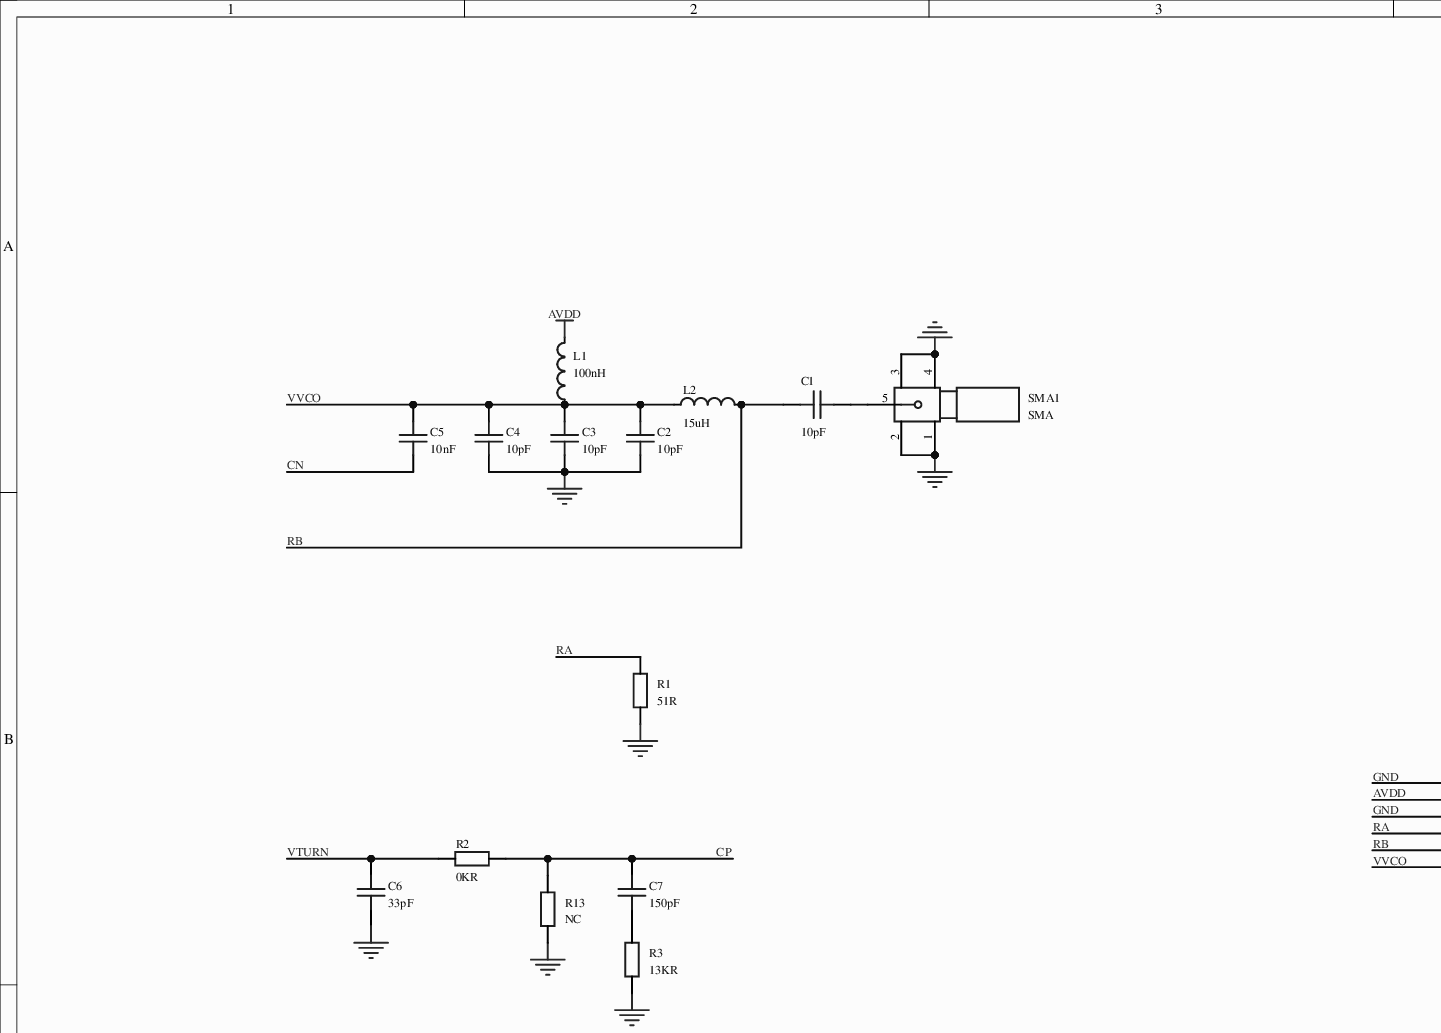
[diagram p0: MISC75048-3.schdoc, top left]
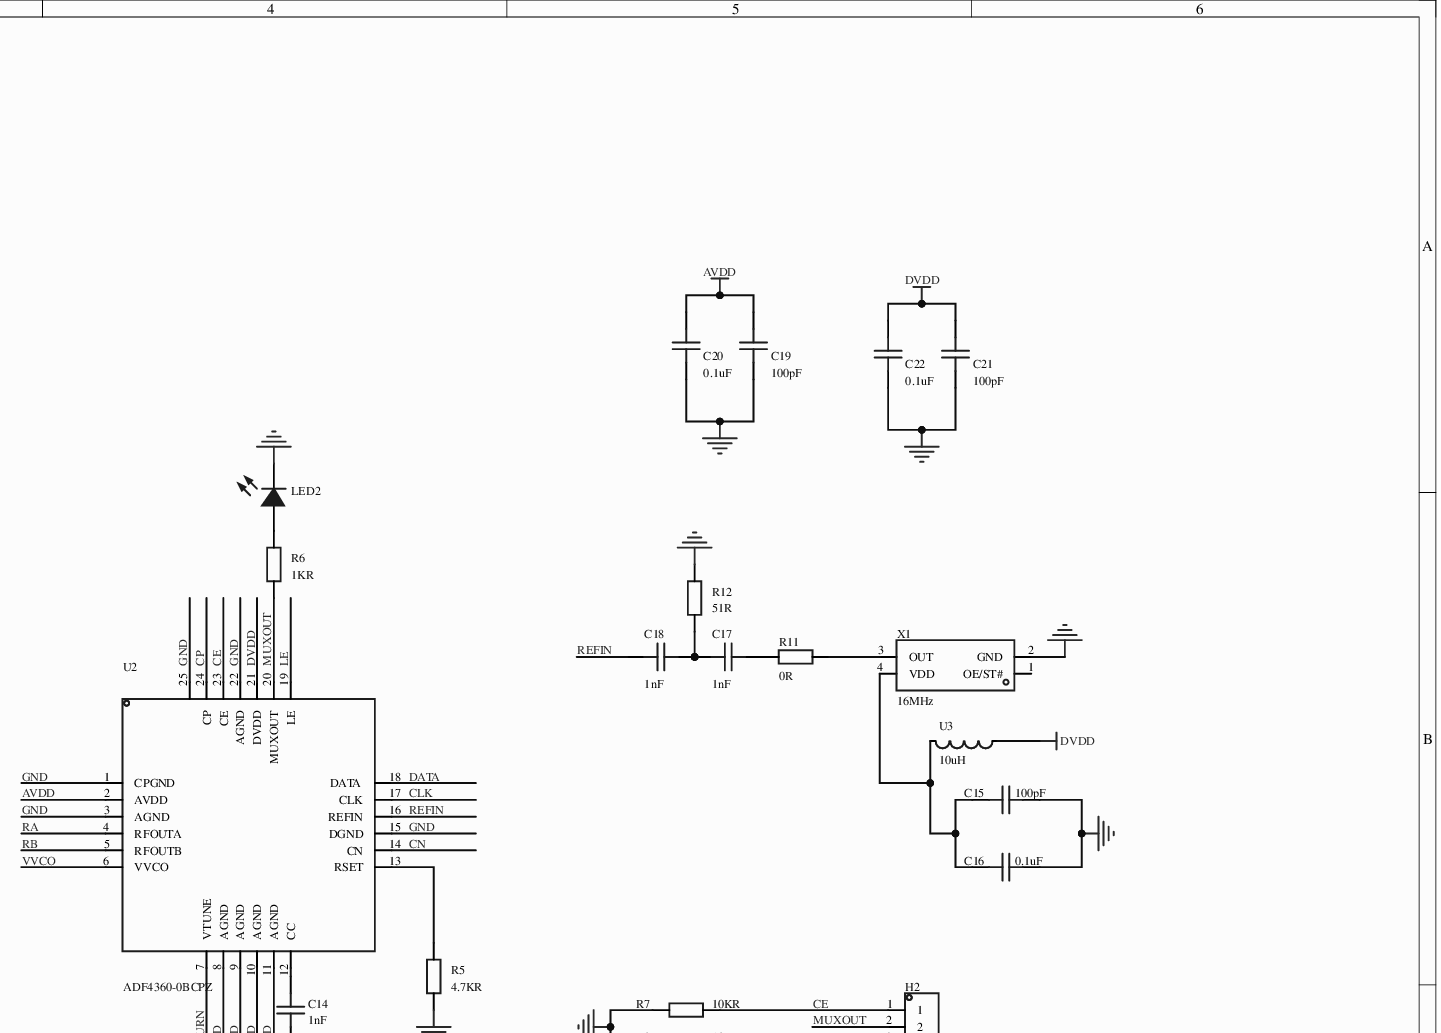
[diagram p1: MISC75048-3.schdoc, top right]
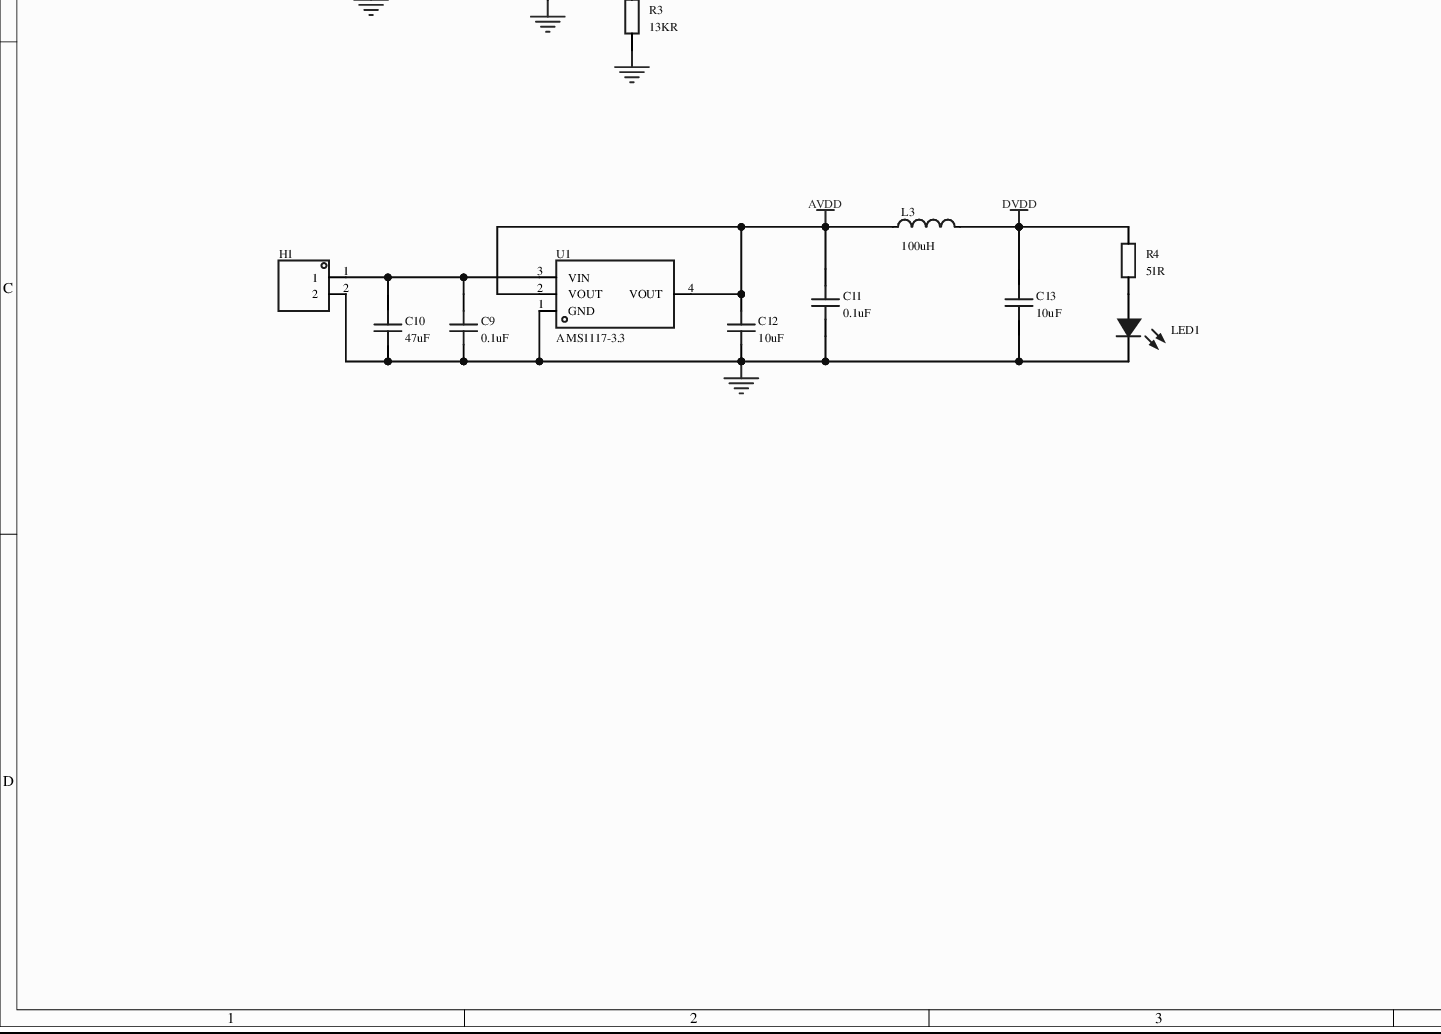
[diagram p2: MISC75048-3.schdoc, bottom left]
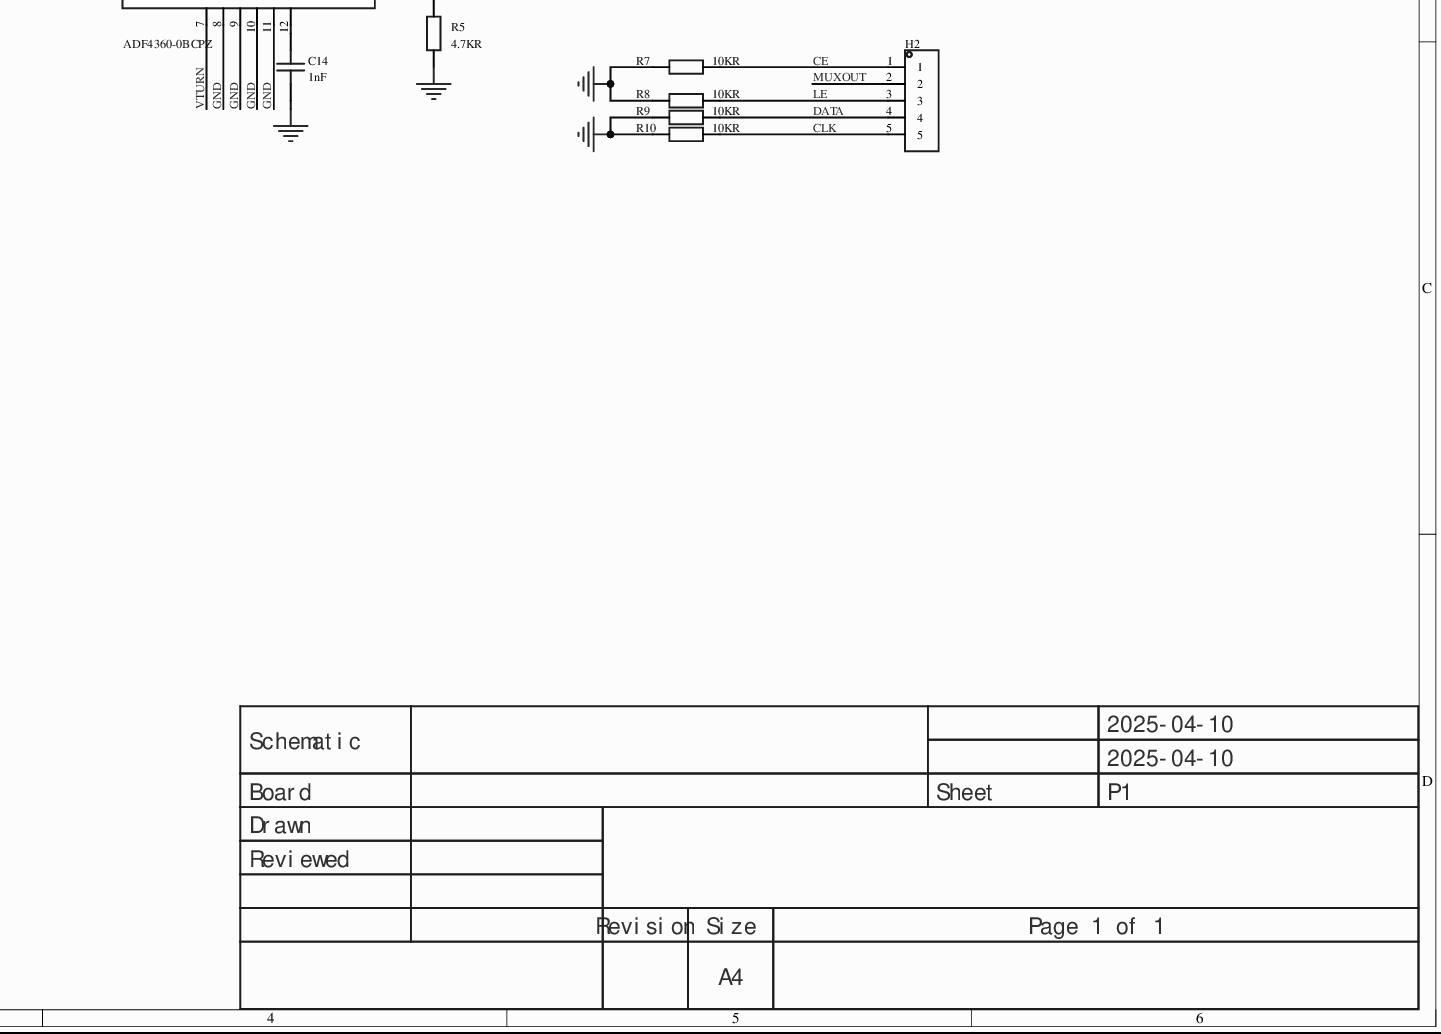
[diagram p3: MISC75048-3.schdoc, bottom right]
# Altium project MISC75048-2.PrjPcb
1 sheet, 46 parts. Net scope: global (net labels, ports and power ports of the same name join across sheets).
Board file: MISC75048.pcbdoc

## Sheet MISC75048-3.schdoc
size 420 x 297 mm; Version: V1.0; @Project Name: MISC75048; @Page Count: 1; @Update Date: 2025-04-10; @Create Date: 2025-04-10; @Schematic Name: MISC75048; @Page No: 1; @Create Time: 22:21:49; @Update Time: 22:48:33; @Board Name: MISC75048

### Parts
C1  10pF  [C0603]
C2  10pF  [C0603]
C3  10pF  [C0603]
C4  10pF  [C0603]
C5  10nF  [C0603]
C6  33pF  [C0603]
C7  150pF  [C0603]
C9  0.1uF  [C0603]
C10  47uF  [C0603]
C11  0.1uF  [C0603]
C12  10uF  [C0603]
C13  10uF  [C0603]
C14  1nF  [C0603]
C15  100pF  [C0603]
C16  0.1uF  [C0603]
C17  1nF  [C0603]
C18  1nF  [C0603]
C19  100pF  [C0603]
C20  0.1uF  [C0603]
C21  100pF  [C0603]
C22  0.1uF  [C0603]
H1  (no value)  [HDR-TH_2P-P2.54-V-M-1]
H2  (no value)  [HDR-TH_5P-P2.54-V-M]
L1  100nH  [L0805]
L2  15uH  [IND-SMD_L8.5-W8.0-LS9.5_ZEYH0850-15UH]
L3  100uH  [IND-SMD_L4.0-W4.0_SWPA4018S]
LED1  (no value)  [LED_0603]
LED2  (no value)  [LED_0603]
R1  51R  [R0603]
R2  0KR  [R0603]
R3  13KR  [R0603]
R4  51R  [R0603]
R5  4.7KR  [R0603]
R6  1KR  [R0603]
R7  10KR  [R0603]
R8  10KR  [R0603]
R9  10KR  [R0603]
R10  10KR  [R0603]
R11  0R  [R0603]
R12  51R  [R0603]
R13  NC  [R0603]
SMA1  SMA  [SMA-SMD_BWSMA-KE-P001]
U1  AMS1117-3.3  [SOT-223-3_L6.5-W3.4-P2.30-LS7.0-BR]
U2  ADF4360-0BCPZ  [LFCSP-24_L4.0-W4.0-P0.50-BL-EP2.3]
U3  10uH  [IND-SMD_L4.0-W4.0_LVF404015]
X1  16MHz  [OSC-SMD_4P-L7.0-W5.0-BL]

### Nets
AVDD: C11.2 C12.2 C19.2 C20.2 L1.2 L3.1 U1.2(VOUT) U1.4(VOUT) U2.2(AVDD)
DVDD: C13.2 C21.2 C22.2 L3.2 R4.2 U2.21(DVDD) U3.1
GND: C2.1 C3.1 C4.1 C6.1 C9.1 C10.1 C11.1 C12.1 C13.1 C14.1 C15.1 C16.1 C19.1 C20.1 C21.1 C22.1 H1.2 LED1.1(C) LED2.1(C) R1.1 R3.2 R5.1 R7.2 R8.2 R9.2 R10.2 R12.2 R13.2 SMA1.1 SMA1.2 SMA1.3 SMA1.4 U1.1(GND) U2.1(CPGND) U2.3(AGND) U2.8(AGND) U2.9(AGND) U2.10(AGND) U2.11(AGND) U2.15(DGND) U2.22(AGND) U2.25 X1.2(GND)
CE: H2.1 R7.1 U2.23(CE)
CLK: H2.5 R10.1 U2.17(CLK)
CN: C5.1 U2.14(CN)
CP: C7.2 R2.1 R13.1 U2.24(CP)
DATA: H2.4 R9.1 U2.18(DATA)
LE: H2.3 R8.1 U2.19(LE)
MUXOUT: H2.2 R6.2 U2.20(MUXOUT)
RA: R1.2 U2.4(RFOUTA)
RB: C1.1 L2.2 U2.5(RFOUTB)
REFIN: C18.2 U2.16(REFIN)
VTURN: C6.2 R2.2 U2.7(VTUNE)
VVCO: C2.2 C3.2 C4.2 C5.2 L1.1 L2.1 U2.6(VVCO)
NetC1_2: C1.2 SMA1.5
NetC7_1: C7.1 R3.1
NetC9_2: C9.2 C10.2 H1.1 U1.3(VIN)
NetC14_2: C14.2 U2.12(CC)
NetC15_2: C15.2 C16.2 U3.2 X1.4(VDD)
NetC17_1: C17.1 R11.1
NetC17_2: C17.2 C18.1 R12.1
NetLED1_2: LED1.2(A) R4.1
NetLED2_2: LED2.2(A) R6.1
NetR5_2: R5.2 U2.13(RSET)
NetR11_2: R11.2 X1.3(OUT)

Not connected (* = marked no-connect by the designer): X1 1(OE/ST#)*

### Notes on the sheet
- 2025-04-10
- Schematic
- Board
- Sheet
- P1
- Drawn
- Reviewed
- Revision
- Size
- A4
- Page 1 of 1

### Library data of the parts
C1-C7 C9-C22 = CAP_0603: ConvertToPcb: yes; SymbolName: CapAcitance; ModelId: ac125912035d415993ca9572d50418b1; ModelName: C0603_L1.6-W0.8-H0.8; ModelTransform: 62.992,31.496,0,0,0,0,0,0,0; Device: CAP_0603; AddInBom: yes; Supplier Footprint: 0603; FootprintName: C0603
  C1-C4: Value: 10pF
  C5: Value: 10nF
  C6: Value: 33pF
  C7: Value: 150pF
  C9 C11 C16 C20 C22: Value: 0.1uF
  C10: Value: 47uF
  C12 C13: Value: 10uF
  C14 C17 C18: Value: 1nF
  C15 C19 C21: Value: 100pF
H1 = HDR-M_2.54_1x2P: Symbol: 210S-1*2P L=11.6MMGold-plated black; ConvertToPcb: yes; ModelId: 79b2e9f2d70a4d68a1b7098f27c6d4c5; ModelName: HDR-M-2.54_1x2; ModelTransform: 200,100,0,0,0,0,0,0,-118.11; Device: HDR-M_2.54_1x2P; AddInBom: yes; SupplierPart: C124375; Supplier Footprint: 插件; FootprintName: HDR-TH_2P-P2.54-V-M-1
H2 = HDR-M_2.54_1x5P: Symbol: MTP125-1105S1; ConvertToPcb: yes; ModelId: 47d466e4a34f4fc5bc626cf773a24dd5; ModelName: HDR-TH_5P-P2.54-M-LI-1X5P; ModelTransform: 499.999,100,0,0,0,0,0,0,-118.11; Device: HDR-M_2.54_1x5P; AddInBom: yes; SupplierPart: C358687; Supplier Footprint: 插件; FootprintName: HDR-TH_5P-P2.54-V-M
L1 = SDFL2012LR10KTF: Inductance: 100nH; Tolerance: ±10%; Rated current: 250mA; Saturation current (Isat): -; DC resistance (DCR): 300mΩ;; Manufacturer: Sunlord(顺络); AddInBom: yes; ModelId: 37a81e68749a4138bd2dfa6897b24b85; ModelName: R0805_L2.0-W1.3-H0.6; ModelTransform: 78.74,51.181,0,0,0,0,0,0.001,0; Symbol: SDFL2012LR10KTF; Device: SDFL2012LR10KTF; LCSC Part Name: 100nH ±10%; SupplierPart: C74321; ManufacturerPart: SDFL2012LR10KTF; Supplier Footprint: 0805; Datasheet: example.com/upload/public/pdf/source/20231027/097A17DDB71564CE812E62F0F80142C9.pdf; Supplier: LCSC; ConvertToPcb: yes; FootprintName: L0805; Value: 100nH; Rated Current: 250mA; Saturation Current (Isat): -; DC Resistance (DCR): 300mΩ; Q @ Freq: -; Frequency - Self Resonant: -; Ratings: -
L2 = ZEYH0850-15UH: Inductance: 15uH; Tolerance: ±20%; Rated current: 5A; Saturation current (Isat): 9A; Type: molded integrated inductor;; Manufacturer: ZE(增益); AddInBom: yes; DC Resistance(DCR): 47mΩ; Symbol: ZEYH0850-15UH; Device: ZEYH0850-15UH; LCSC Part Name: 15uH ±20% 9A; SupplierPart: C45986904; ManufacturerPart: ZEYH0850-15UH; Supplier Footprint: SMD,8.5x8mm; Datasheet: example.com/upload/public/pdf/source/20250227/8D198FBC2D11620209AF2814C1FD1B5F.pdf; Supplier: LCSC; ConvertToPcb: yes; FootprintName: IND-SMD_L8.5-W8.0-LS9.5_ZEYH0850-15UH; Value: 15uH; Current Rating: 5A; Current - Saturation(Isat): 9A; Type: Molded integrated inductor
L3 = SWPA4012S101MT: Inductance: 100uH; Tolerance: ±20%; Rated current: 250mA; Saturation current (Isat): 250mA; Type: -;; Manufacturer: Sunlord(顺络); AddInBom: yes; ModelId: a0312046766d423b9f3ce3b362dc752d; ModelName: IND-SMD_L4.0-W4.0-H3.0; ModelTransform: 157.48,158.267,0,90,0,0,0,0,0; DC Resistance(DCR): 2.21Ω; Symbol: SWPA4012S101MT; Device: SWPA4012S101MT; LCSC Part Name: 100uH ±20% 250mA; SupplierPart: C55384; ManufacturerPart: SWPA4012S101MT; Supplier Footprint: SMD,4x4mm; JLCPCB Part Class: Extended library; Datasheet: example.com/upload/public/pdf/source/20231024/317626D2AA2F8AB4113C1875E432E6E1.pdf; Supplier: LCSC; ConvertToPcb: yes; FootprintName: IND-SMD_L4.0-W4.0_SWPA4018S; Value: 100uH; Rated Current: 250mA; Current - Saturation(Isat): 250mA; Type: -; Ratings: -
LED1 LED2 = LED_0603-B: Symbol: LED_B; Convert to PCB: yes; 3D Model: eb8d964598f24248affda46f619856c5; 3D Model Transform: 63.1,31.6,23.7,0,0,0,0,0,0; ModelName: LED-0603_B; Device: LED_0603-B; Add into BOM: yes; Supplier Footprint: 0603; FootprintName: LED_0603
R1-R13 = Res_0603: ConvertToPcb: yes; SymbolName: Resistor; ModelId: fc143cca1e79419f9cd78b61e9279f08; ModelTransform: 31.8897,63.7794,0,90,0,0,0,0,0; Device: Res_0603; AddInBom: yes; Supplier Footprint: 0603; FootprintName: R0603; ModelName: R0603
  R1 R4 R12: Value: 51R
  R2: Value: 0KR
  R3: Value: 13KR
  R5: Value: 4.7KR
  R6: Value: 1KR
  R7-R10: Value: 10KR
  R11: Value: 0R
  R13: Value: NC
SMA1 = SMA: Symbol: SMA_C9900018296; AddInBom: yes; ModelId: 45bafb7576014fe1be3aebd244b0ca8e; ModelName: SMA-TH_5P-L6.5-W6.5-H9.5_BWSMA-KE-P001; ModelTransform: 255.905,255.905,0,180,0,90,-23.62,0,17.717; Device: SMA; LCSC Part Name: SMA; SupplierPart: C9900018296; ManufacturerPart: SMA; Supplier Footprint: SMA-SMD_BWSMA-KE-P001; JLCPCB Part Class: Extended library; Supplier: LCSC; ConvertToPcb: yes; FootprintName: SMA-SMD_BWSMA-KE-P001
U1 = AMS1117-3.3_C6186: Output type: fixed; Operating voltage: -; Output voltage: 3.3V; Output current: 1A; Power supply rejection ratio (PSRR): 72dB@(120Hz); Output polarity: positive;; Manufacturer: AMS; AddInBom: yes; ModelId: 925194bf9823436183a3e0b978a8d076; ModelName: SOT-223-4P_L6.5-W3.5-H1.6-LS7.0-P2.30; ModelTransform: 279.89794,255.905,0,180,0,0,-3.9385,-0.0005,0; Voltage Dropout: 1.3V@(800mA); Number of Outputs: 1; Symbol: AMS1117-3.3; Device: AMS1117-3.3_C6186; LCSC Part Name: 输出3.3V 1A; SupplierPart: C6186; ManufacturerPart: AMS1117-3.3; Supplier Footprint: SOT-223; Datasheet: example.com/upload/public/pdf/source/20180727/C6186_7A095716F0823C02F1997A905E26C086.pdf; Supplier: LCSC; ConvertToPcb: yes; FootprintName: SOT-223-3_L6.5-W3.4-P2.30-LS7.0-BR; Output Type: Fixed; Voltage - Supply: -; Output Voltage: 3.3V; Output Current: 1A; Power Supply Rejection Ratio (PSRR): 72dB@(120Hz); standby current: -; Noise: -; Features: Overcurrent protection (OCP); Thermal shutdown (TSD); Operating Temperature: -; Output Configuration: Positive
U2 = ADF4360-0BCPZ: Maximum output frequency: 2.725GHz;; Manufacturer: ADI(亚德诺); AddInBom: yes; ModelId: fa197dd414874ad2bc21045e91d88c96; ModelName: LFCSP-24_L4.0-W4.0-H0.8-P0.50; ModelTransform: 157.48,157.48,0,90,0,0,0,0,0; Supply Voltage: 3V~3.6V; Symbol: ADF4360-0BCPZ; Device: ADF4360-0BCPZ; LCSC Part Name: 集成式整数N分频合成器/VCO输出频率范围为2400 MHz至2725 MHz; SupplierPart: C209527; ManufacturerPart: ADF4360-0BCPZ; Supplier Footprint: LFCSP-24(4x4); JLCPCB Part Class: Extended library; Datasheet: example.com/upload/public/pdf/source/20180524/C208221_3F274C0A6513F969727BEBB74B9FE267.pdf; Supplier: LCSC; ConvertToPcb: yes; FootprintName: LFCSP-24_L4.0-W4.0-P0.50-BL-EP2.3; Output Frequency (Max): 2.725GHz; Operating Temperatue: -40℃~+85℃
U3 = 10uH: Symbol: 10UH_C9900025245; AddInBom: yes; ModelId: e5ace3c9dad0416cb941f601801b3ad2; ModelName: IND-SMD_L4.0-W4.0-H1.5_LVF404015; ModelTransform: 157.48,157.48,0,90,0,0,0,0,0; Device: 10uH; LCSC Part Name: 10uH; SupplierPart: C9900025245; ManufacturerPart: 10uH; Supplier Footprint: IND-SMD; JLCPCB Part Class: Extended library; Supplier: LCSC; ConvertToPcb: yes; FootprintName: IND-SMD_L4.0-W4.0_LVF404015
X1 = SG-8002CA 16.000000MHz PCM: Frequency: 16MHz; Frequency stability: ±100ppm; Operating voltage: 2.7V~3.6V;; Manufacturer: EPSON(爱普生); AddInBom: yes; ModelId: 2fc04ec2295f4b92bdb5570bebe319d8; ModelName: OSC-SMD_4P-L7.0-W5.0-H1.3; ModelTransform: 275.59,196.85,0,0,0,0,0,0,0; Symbol: SG-8002CA 16.000000MHZ PCM; Device: SG-8002CA 16.000000MHz PCM; LCSC Part Name: 16MHz ±100ppm 2.7V~3.6V; SupplierPart: C390297; ManufacturerPart: SG-8002CA 16.000000MHz PCM; Supplier Footprint: SMD7050-4P; Datasheet: example.com/upload/public/pdf/source/20190725/C390312_9B963BCCDCB461DF88AB8B71FD2CB2DB.pdf; Supplier: LCSC; ConvertToPcb: yes; FootprintName: OSC-SMD_4P-L7.0-W5.0-BL; Value: 16MHz; Frequency Stability: ±100ppm; Voltage - Supply: 2.7V~3.6V; Operating Temperature: -40℃~+85℃